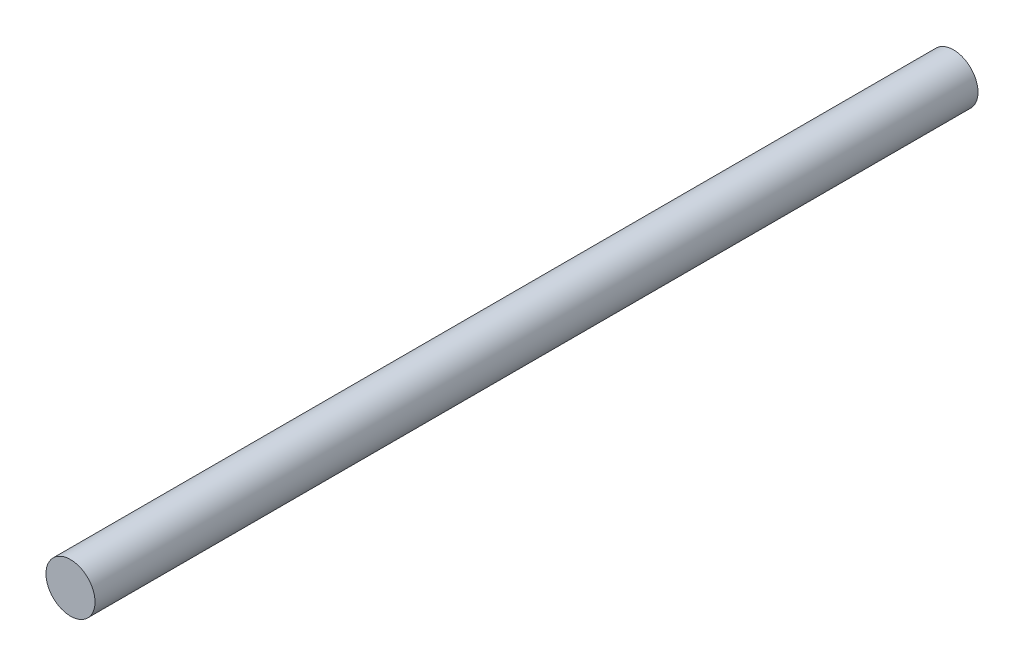
from build123d import *

# Parameters (mm, degrees)
SKETCH_1_R      = 4
EXTRUDE_1_DEPTH = 72


with BuildPart() as part:
    # 草图1 → 凸台-拉伸1 (new, symmetric)
    with BuildSketch(Plane.XY):
        Circle(SKETCH_1_R)
    extrude(amount=EXTRUDE_1_DEPTH, both=True)


solid = part.part
